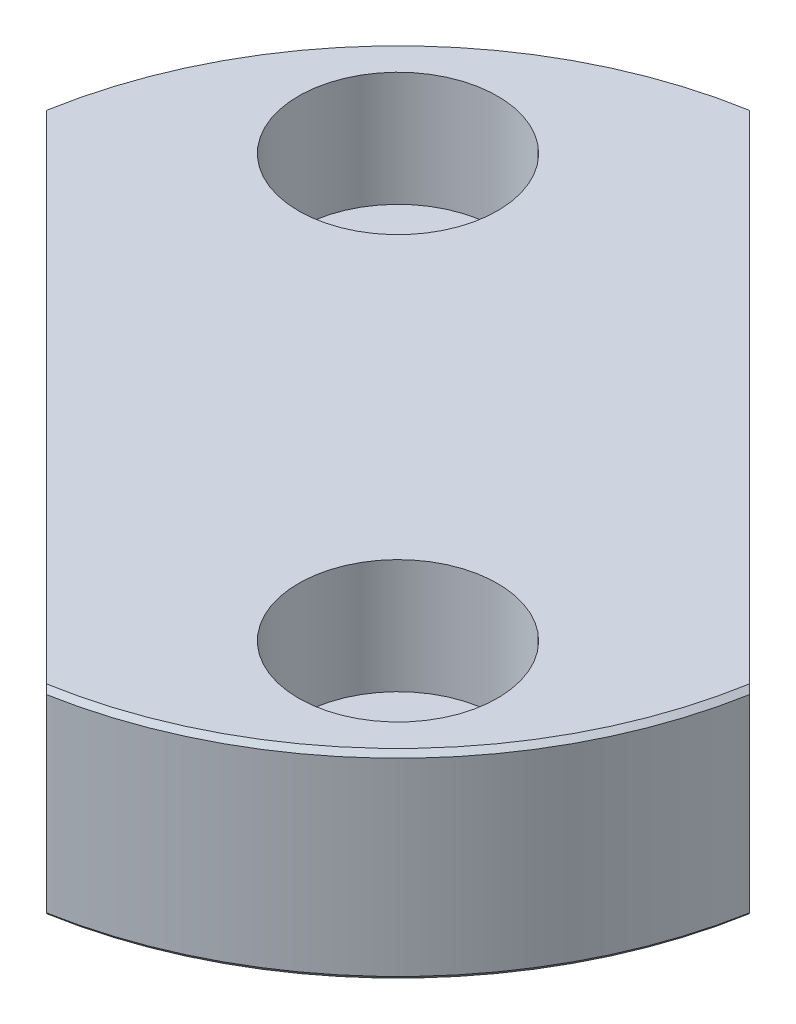
from build123d import *

# Parameters (mm, degrees)
G1_8_TAPPED_HOLE1_D                               = 8.8
HOLE_SIZE_BASED_ON_SOCKET_HEAD_CAP_SC_D           = 4.8
HOLE_SIZE_BASED_ON_SOCKET_HEAD_CAP_SC_CBORE_D     = 8
HOLE_SIZE_BASED_ON_SOCKET_HEAD_CAP_SC_CBORE_DEPTH = 4.6
FILLET1_R                                         = 0.2
CHAMFER1_SIZE                                     = 0.2
CHAMFER2_SIZE                                     = 0.5
CUT_EXTRUDE1_DEPTH                                = 35.474628352
SKETCH8_R                                         = 15
CUT_EXTRUDE2_DEPTH                                = 30.145808143
SKETCH9_R                                         = 7
BOSS_EXTRUDE1_DEPTH                               = 8


with BuildPart() as part:
    # Sketch2 → Revolve1 (revolve)
    with BuildSketch(Plane.XY, mode=Mode.PRIVATE) as revolve1_sk:
        Polygon((0, 24), (-17.5, 24), (-17.5, 16), (-6.75, 16), (-6.75, 0), (0, 0), align=None)
    revolve(revolve1_sk.sketch.rotate(Axis((0, 0, 0), (0, 1, 0)), 270), axis=Axis((0, 0, 0), (0, 1, 0)))

    # G1/8 Tapped Hole1 (through all)
    with Locations(Plane.ZX.offset(24)):
        with Locations((0, 0)):
            Hole(G1_8_TAPPED_HOLE1_D / 2)

    # Hole Size (% based on) Socket Head Cap Screw Type 1 (through all)
    with Locations(Plane(origin=(-8.485281374, 24, -8.485281374), x_dir=(0, 0, 1), z_dir=(0, 1, 0))):
        with Locations((0, 0), (16.970562748, 16.970562748)):
            CounterBoreHole(HOLE_SIZE_BASED_ON_SOCKET_HEAD_CAP_SC_D / 2, HOLE_SIZE_BASED_ON_SOCKET_HEAD_CAP_SC_CBORE_D / 2, HOLE_SIZE_BASED_ON_SOCKET_HEAD_CAP_SC_CBORE_DEPTH)

    # Fillet1
    fillet1_edges = [part.edges().sort_by_distance(p)[0] for p in [
        (0, 16, 6.75),
    ]]
    fillet(fillet1_edges, radius=FILLET1_R)

    # Chamfer1
    chamfer1_edges = [part.edges().sort_by_distance(p)[0] for p in [
        (0, 0, 6.75),
        (0, 16, 17.5),
        (0, 24, 17.5),
    ]]
    chamfer(chamfer1_edges, length=CHAMFER1_SIZE)

    # Chamfer2
    chamfer2_edges = [part.edges().sort_by_distance(p)[0] for p in [
        (0, 24, 4.4),
        (0, 0, 4.4),
    ]]
    chamfer(chamfer2_edges, length=CHAMFER2_SIZE)

    # Sketch7 → Cut-Extrude1 (cut, through all)
    with BuildSketch(Plane(origin=(0, 24, 0), x_dir=(1, 0, 0), z_dir=(0, 1, 0))):
        with BuildLine():
            Line((2.911166407, -17.053302031), (-17.053302031, 2.911166407))
            ThreePointArc((-17.053302031, 2.911166407), (-12.232947315, -12.232947315), (2.911166407, -17.053302031))
        make_face()
        with BuildLine():
            ThreePointArc((17.3, 0), (11.156317071, 13.222200627), (-2.911166407, 17.053302031))
            Line((-2.911166407, 17.053302031), (17.053302031, -2.911166407))
            ThreePointArc((17.053302031, -2.911166407), (17.238215179, -1.460800272), (17.3, 0))
        make_face()
        with BuildLine():
            Line((-17.053302031, 2.911166407), (-17.226115818, 3.083980194))
            ThreePointArc((-17.226115818, 3.083980194), (-12.374368671, -12.374368671), (3.083980194, -17.226115818))
            Line((3.083980194, -17.226115818), (2.911166407, -17.053302031))
            ThreePointArc((2.911166407, -17.053302031), (-12.232947315, -12.232947315), (-17.053302031, 2.911166407))
        make_face()
        with BuildLine():
            ThreePointArc((17.5, 0), (11.23121424, 13.42050024), (-3.083980194, 17.226115818))
            Line((-3.083980194, 17.226115818), (-2.911166407, 17.053302031))
            ThreePointArc((-2.911166407, 17.053302031), (11.156317071, 13.222200627), (17.3, 0))
            ThreePointArc((17.3, 0), (17.238215179, -1.460800272), (17.053302031, -2.911166407))
            Line((17.053302031, -2.911166407), (17.226115818, -3.083980194))
            ThreePointArc((17.226115818, -3.083980194), (17.431394477, -1.548058977), (17.5, 0))
        make_face()
    extrude(amount=-CUT_EXTRUDE1_DEPTH, mode=Mode.SUBTRACT)

    # Sketch8 → Cut-Extrude2 (cut, through all)
    with BuildSketch(Plane.XZ.offset(-16)):
        Circle(SKETCH8_R)
    extrude(amount=CUT_EXTRUDE2_DEPTH, mode=Mode.SUBTRACT)

    # Sketch9 → Boss-Extrude1 (add)
    with BuildSketch(Plane.XZ.offset(-16)):
        Circle(SKETCH9_R)
    extrude(amount=-BOSS_EXTRUDE1_DEPTH)


solid = part.part
